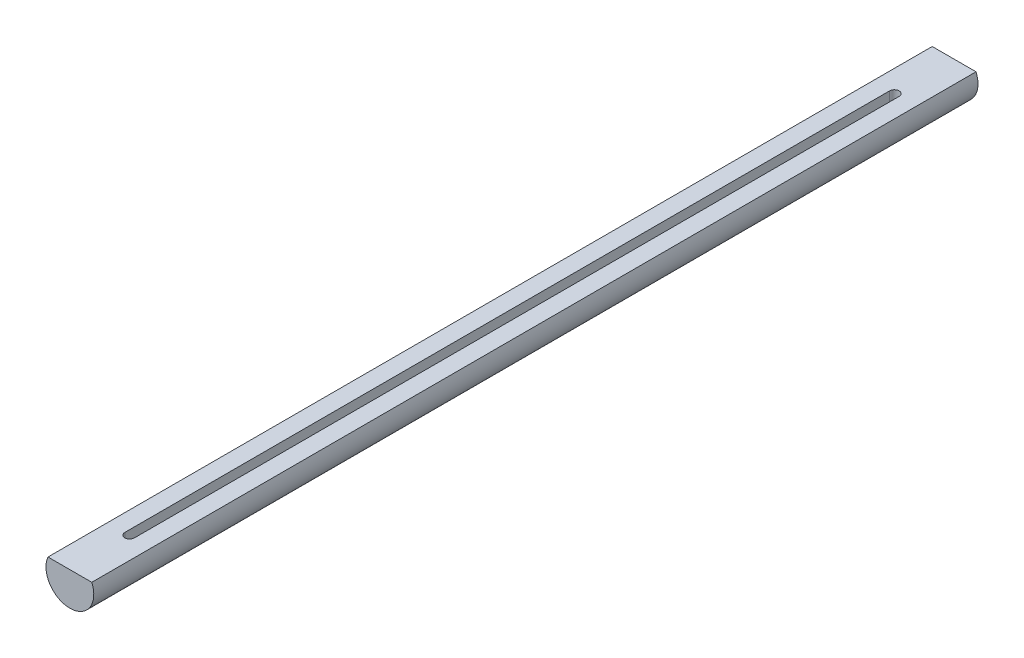
from build123d import *

# Parameters (mm, degrees)
SKETCH_3_R          = 10
EXTRUDE_3_DEPTH     = 185
CUT_EXTRUDE_1_DEPTH = 12.5
SKETCH_5_W          = 370
SKETCH_5_H          = 20
CUT_EXTRUDE_2_DEPTH = 10


with BuildPart() as part:
    # 草图3 → 凸台-拉伸3 (new, symmetric)
    with BuildSketch(Plane.XY):
        Circle(SKETCH_3_R)
    extrude(amount=EXTRUDE_3_DEPTH, both=True)

    # 草图4 → 切除-拉伸1 (cut, symmetric)
    with BuildSketch(Plane(origin=(0, 0, 0), x_dir=(1, 0, 0), z_dir=(0, 1, 0))):
        with BuildLine():
            Line((-2, -160), (-2, 160))
            ThreePointArc((-2, 160), (0, 162), (2, 160))
            Line((2, 160), (2, -160))
            ThreePointArc((2, -160), (0, -162), (-2, -160))
        make_face()
    extrude(amount=CUT_EXTRUDE_1_DEPTH, both=True, mode=Mode.SUBTRACT)

    # 草图5 → 切除-拉伸2 (cut, symmetric)
    with BuildSketch(Plane(origin=(0, 0, 0), x_dir=(0, 0, -1), z_dir=(1, 0, 0))):
        with Locations((0, 14)):
            Rectangle(SKETCH_5_W, SKETCH_5_H)
    extrude(amount=CUT_EXTRUDE_2_DEPTH, both=True, mode=Mode.SUBTRACT)


solid = part.part
